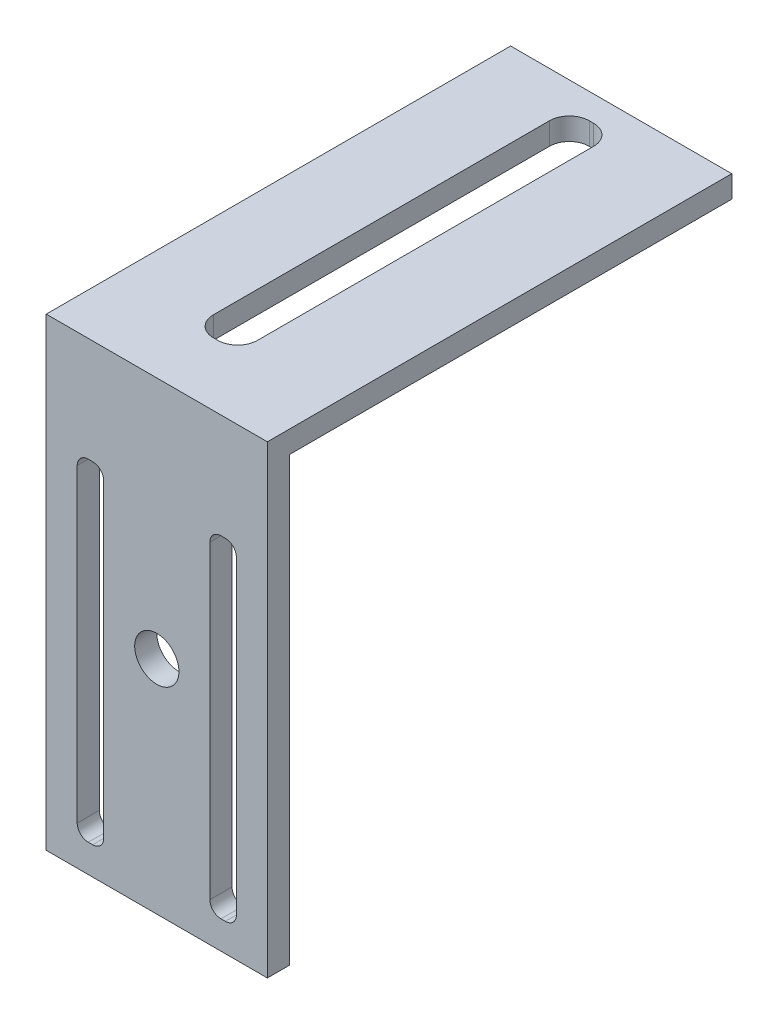
from build123d import *

# Parameters (mm, degrees)
SKETCH1_W                = 50
SKETCH1_H                = 100
BOSS_EXTRUDE1_DEPTH      = 5
CUT_EXTRUDE1_DEPTH       = 10
SKETCH3_R                = 5
CUT_EXTRUDE2_DEPTH       = 10
BOSS_EXTRUDE2_DEPTH      = 100
BOSS_EXTRUDE2_DEPTH_BACK = 5
SKETCH4_W                = 50
SKETCH4_H                = 5
CUT_EXTRUDE3_DEPTH       = 80


with BuildPart() as part:
    # Sketch1 → Boss-Extrude1 (new body)
    with BuildSketch(Plane.XY):
        Rectangle(SKETCH1_W, SKETCH1_H)
    extrude(amount=BOSS_EXTRUDE1_DEPTH)

    # Sketch2 → Cut-Extrude1 (cut)
    with BuildSketch(Plane.XY.offset(5)):
        with BuildLine():
            Line((-14.5, -43.655057898), (-15.5, -43.655057898))
            ThreePointArc((-15.5, -43.655057898), (-17.267766953, -42.922824851), (-18, -41.155057898))
            Line((-18, -41.155057898), (-18, 28.844942102))
            ThreePointArc((-18, 28.844942102), (-17.267766953, 30.612709055), (-15.5, 31.344942102))
            Line((-15.5, 31.344942102), (-14.5, 31.344942102))
            ThreePointArc((-14.5, 31.344942102), (-12.732233047, 30.612709055), (-12, 28.844942102))
            Line((-12, 28.844942102), (-12, -41.155057898))
            ThreePointArc((-12, -41.155057898), (-12.732233047, -42.922824851), (-14.5, -43.655057898))
        make_face()
        with BuildLine():
            Line((15.5, -43.655057898), (14.5, -43.655057898))
            ThreePointArc((14.5, -43.655057898), (12.732233047, -42.922824851), (12, -41.155057898))
            Line((12, -41.155057898), (12, 28.844942102))
            ThreePointArc((12, 28.844942102), (12.732233047, 30.612709055), (14.5, 31.344942102))
            Line((14.5, 31.344942102), (15.5, 31.344942102))
            ThreePointArc((15.5, 31.344942102), (17.267766953, 30.612709055), (18, 28.844942102))
            Line((18, 28.844942102), (18, -41.155057898))
            ThreePointArc((18, -41.155057898), (17.267766953, -42.922824851), (15.5, -43.655057898))
        make_face()
    extrude(amount=-CUT_EXTRUDE1_DEPTH, mode=Mode.SUBTRACT)

    # Sketch3 → Cut-Extrude2 (cut)
    with BuildSketch(Plane.XY.offset(5)):
        Circle(SKETCH3_R)
    extrude(amount=-CUT_EXTRUDE2_DEPTH, mode=Mode.SUBTRACT)

    # Sketch4 → Boss-Extrude2 (add, two sides: drawn at the far end of the back side and taken through both)
    with BuildSketch(Plane(origin=(0, 0, 0), x_dir=(-1, 0, 0), z_dir=(0, 0, -1)).offset(-BOSS_EXTRUDE2_DEPTH_BACK)):
        with Locations((0, 52.5)):
            Rectangle(SKETCH4_W, SKETCH4_H)
    extrude(amount=BOSS_EXTRUDE2_DEPTH + BOSS_EXTRUDE2_DEPTH_BACK)

    # Sketch5 → Cut-Extrude3 (cut)
    with BuildSketch(Plane.XZ.offset(-50)):
        with BuildLine():
            Line((-0.473985761, -94.252877225), (-1.473985761, -94.252877225))
            ThreePointArc((-1.473985761, -94.252877225), (-4.655966276, -92.934857741), (-5.973985761, -89.752877225))
            Line((-5.973985761, -89.752877225), (-5.973985761, -13.752877225))
            ThreePointArc((-5.973985761, -13.752877225), (-4.655966276, -10.57089671), (-1.473985761, -9.252877225))
            Line((-1.473985761, -9.252877225), (-0.473985761, -9.252877225))
            ThreePointArc((-0.473985761, -9.252877225), (2.707994755, -10.57089671), (4.026014239, -13.752877225))
            Line((4.026014239, -13.752877225), (4.026014239, -89.752877225))
            ThreePointArc((4.026014239, -89.752877225), (2.707994755, -92.934857741), (-0.473985761, -94.252877225))
        make_face()
    extrude(amount=-CUT_EXTRUDE3_DEPTH, mode=Mode.SUBTRACT)


solid = part.part
